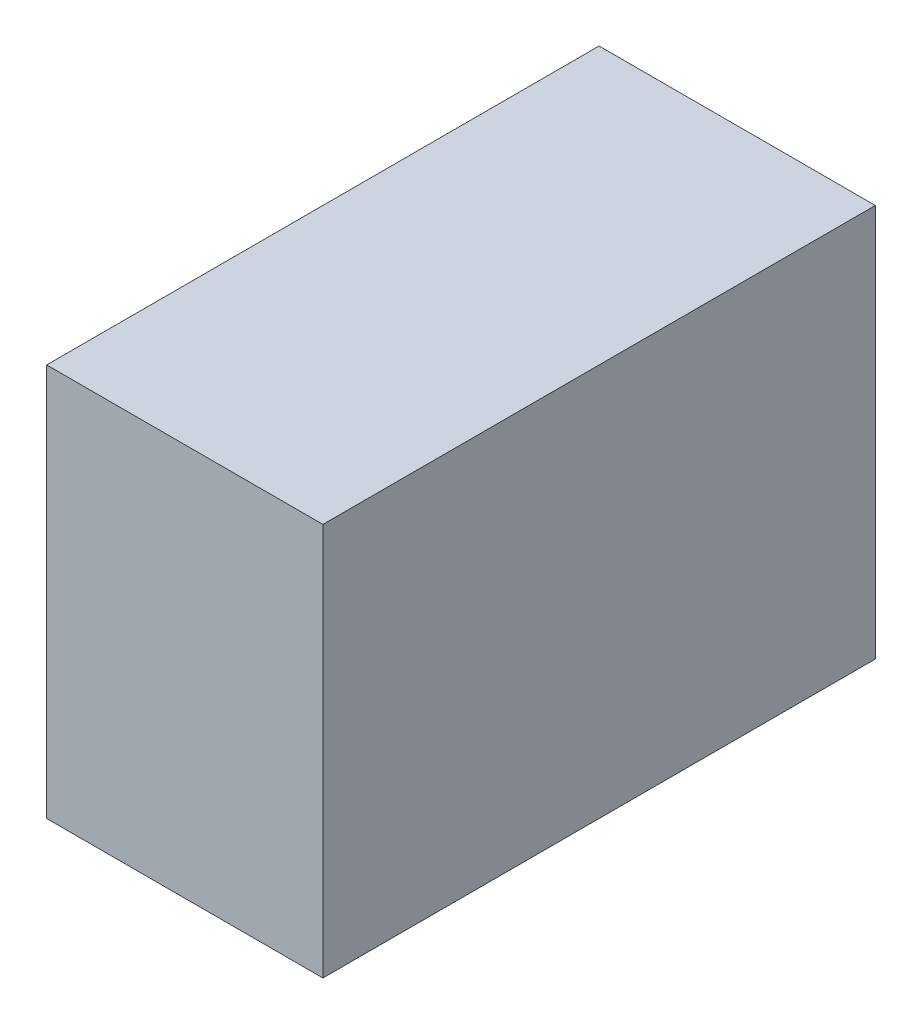
from build123d import *

# Parameters (mm, degrees)
SKETCH_1_W      = 45
SKETCH_1_H      = 90
EXTRUDE_1_DEPTH = 64


with BuildPart() as part:
    # 草图1 → 凸台-拉伸1 (new body)
    with BuildSketch(Plane(origin=(0, 0, 0), x_dir=(1, 0, 0), z_dir=(0, 1, 0))):
        Rectangle(SKETCH_1_W, SKETCH_1_H)
    extrude(amount=EXTRUDE_1_DEPTH)


solid = part.part
